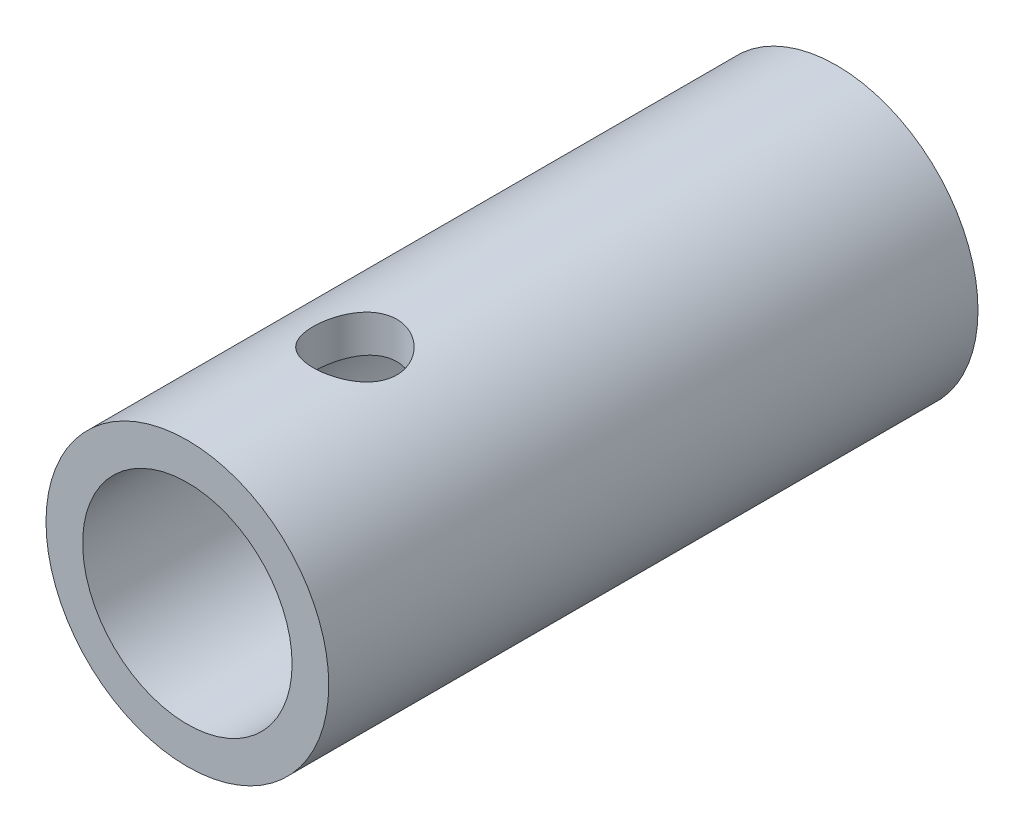
from build123d import *

# Parameters (mm, degrees)
SKETCH1_R           = 13.5
SKETCH1_R_2         = 10
BOSS_EXTRUDE1_DEPTH = 62
SKETCH2_R           = 4
CUT_EXTRUDE1_DEPTH  = 62


with BuildPart() as part:
    # Sketch1 → Boss-Extrude1 (new body)
    with BuildSketch(Plane.XY):
        Circle(SKETCH1_R)
        Circle(SKETCH1_R_2, mode=Mode.SUBTRACT)
    extrude(amount=-BOSS_EXTRUDE1_DEPTH)

    # Sketch2 → Cut-Extrude1 (cut)
    with BuildSketch(Plane(origin=(0, 0, 0), x_dir=(1, 0, 0), z_dir=(0, 1, 0))):
        with Locations(Location((0, 16, 0), (0, 0, 90))):
            Circle(SKETCH2_R)
    extrude(amount=CUT_EXTRUDE1_DEPTH, mode=Mode.SUBTRACT)


solid = part.part
